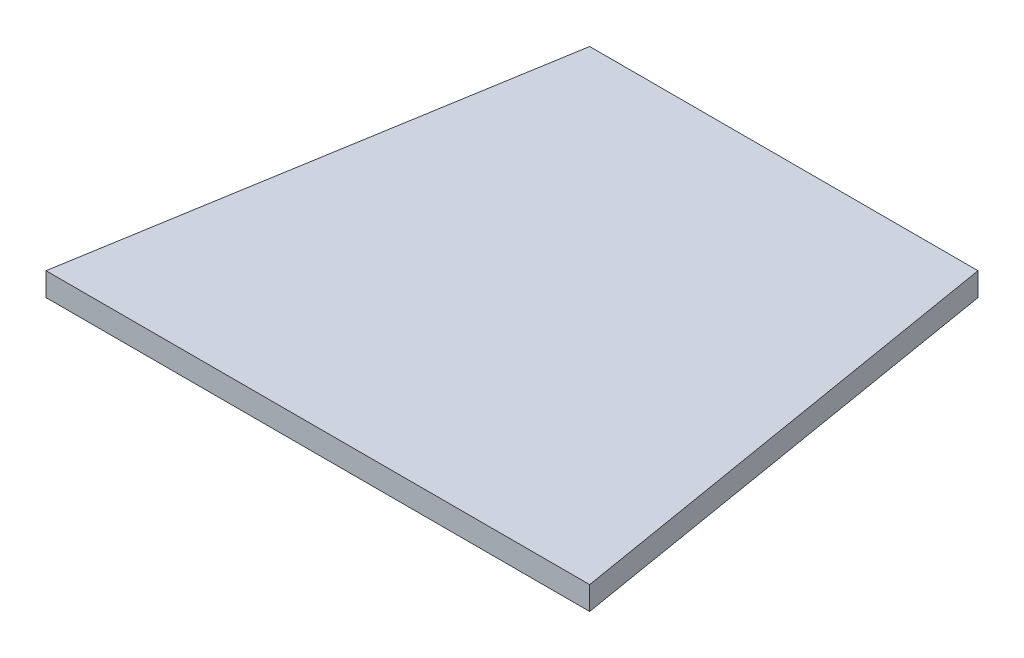
SolidWorks part; units mm, degrees
material "Plain carbon steel"
ref_plane "Front plane" through (0, 0, 0) normal (0, 0, 1) x (1, 0, 0)
ref_plane "Top plane" through (0, 0, 0) normal (0, 1, 0) x (1, 0, 0)
ref_plane "Right plane" through (0, 0, 0) normal (1, 0, 0) x (0, 0, -1)
other "Configuration Table"
sketch "Sketch1" plane through (0, 0, 0) normal (0, 1, 0) x (1, 0, 0)
  line L0 (0, -30) -> (0, 30) construction
  line L1 (-25, 30) -> (25, 30)
  line L2 (-35, -30) -> (35, -30)
  line L3 (-25, 30) -> (-35, -30)
  line L4 (25, 30) -> (35, -30)
  point P4 (0, 0)
  point P8 (0, 30)
  point P11 (0, -30)
  dimension "D1" = 60
  dimension "D2" = 50
  dimension "D3" = 70
extrude "Boss-Extrude1" add sketch "Sketch1" along normal blind 3
